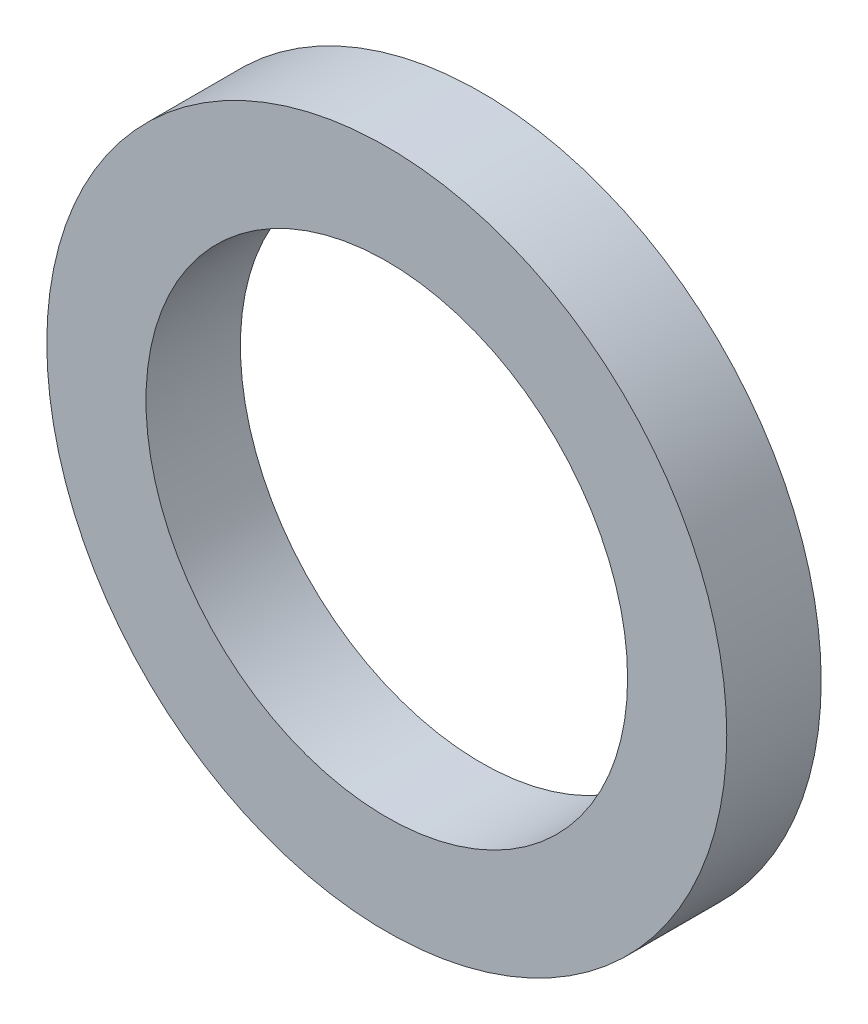
SolidWorks part; units mm, degrees
ref_plane "Front Plane" through (0, 0, 0) normal (0, 0, 1) x (1, 0, 0)
ref_plane "Top Plane" through (0, 0, 0) normal (0, 1, 0) x (1, 0, 0)
ref_plane "Right Plane" through (0, 0, 0) normal (1, 0, 0) x (0, 0, -1)
other "Configuration Table"
sketch "Sketch1" plane through (0, 0, 0) normal (0, 0, 1) x (1, 0, 0)
  circle A0 centre (0, 0) radius 18
  circle A2 centre (0, 0) radius 12.75
  dimension "D1" = 25.5
  dimension "D2" = 36
extrude "Boss-Extrude1" add sketch "Sketch1" along normal blind 5
